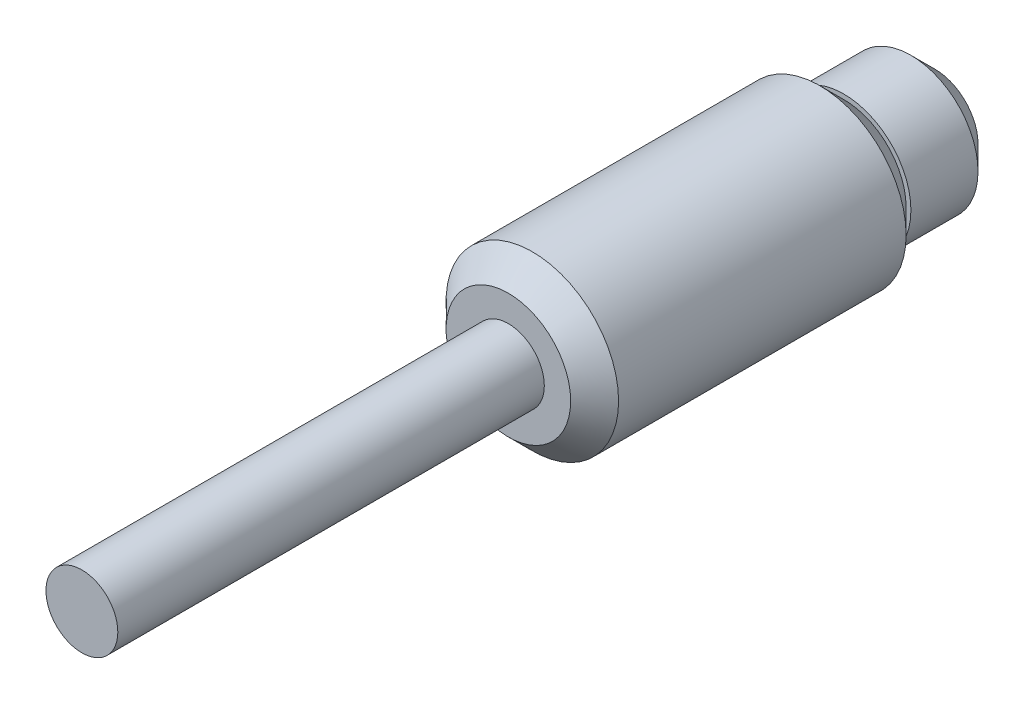
SolidWorks part; units mm, degrees
ref_plane "前视基准面" through (0, 0, 0) normal (0, 0, 1) x (1, 0, 0)
ref_plane "上视基准面" through (0, 0, 0) normal (0, 1, 0) x (1, 0, 0)
ref_plane "右视基准面" through (0, 0, 0) normal (1, 0, 0) x (0, 0, -1)
sketch "草图2" plane through (0, 0, 0) normal (0, 0, 1) x (1, 0, 0)
  circle A0 centre (0, 0) radius 1.8
  dimension "D1" = 3.6
extrude "拉伸1" add sketch "草图2" along normal blind 7
sketch "草图3" plane through (0, 0, 7) normal (0, 0, 1) x (1, 0, 0)
  circle A0 centre (0, 0) radius 0.75
  dimension "D1" = 1.5
extrude "拉伸2" add sketch "草图3" along normal blind 8.9
chamfer "倒角1" distance 0.5 angle 45 1 edges at (1.8, 0, 0)
chamfer "倒角2" distance 0.5 angle 45 1 edges at (1.8, 0, 7)
sketch "草图4" plane through (0, 0, 0) normal (0, 0, -1) x (-1, 0, 0)
  circle A0 centre (0, 0) radius 1.4
  dimension "D1" = 2.8
extrude "拉伸3" add sketch "草图4" along normal blind 1.9
chamfer "倒角3" distance 0.5 angle 45 1 edges at (-1.4, 0, -1.9)
